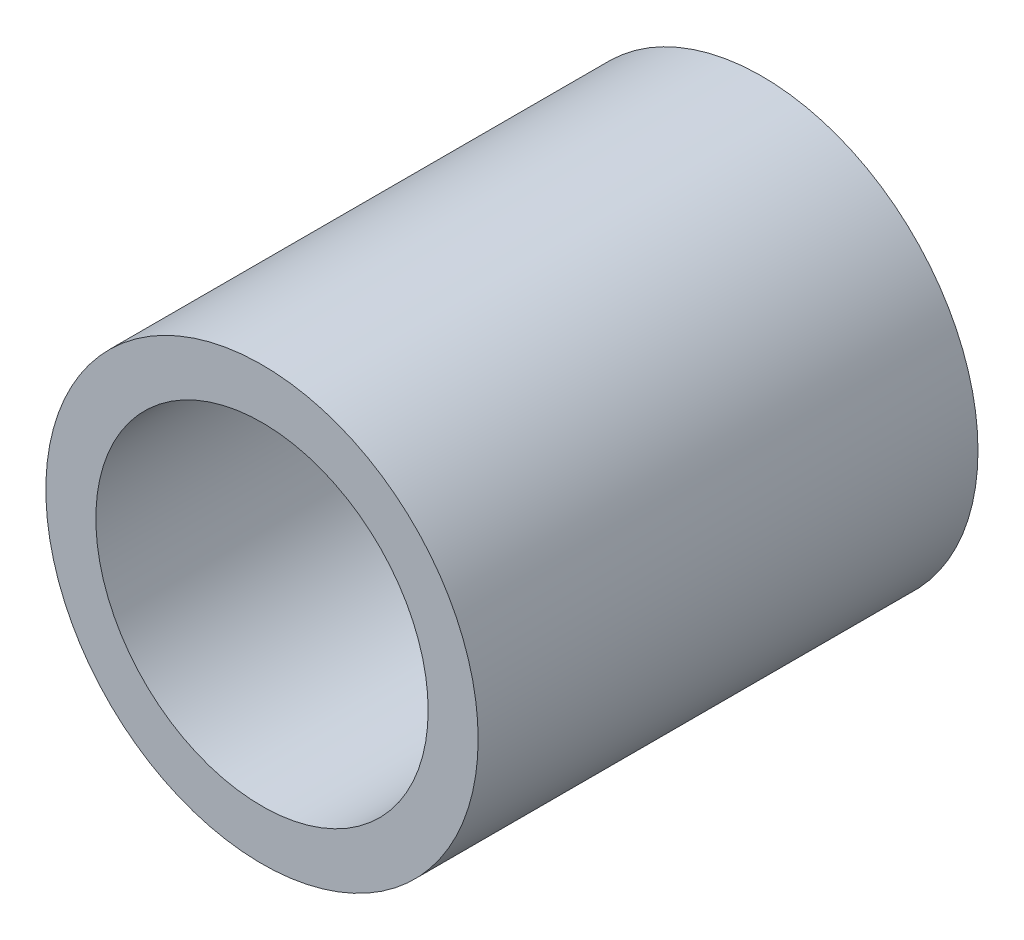
from build123d import *

# Parameters (mm, degrees)
SKETCH1_R           = 8
SKETCH1_R_2         = 6.15
BOSS_EXTRUDE1_DEPTH = 18.5


with BuildPart() as part:
    # Sketch1 → Boss-Extrude1 (new body)
    with BuildSketch(Plane.XY):
        with Locations((100, 71.3)):
            Circle(SKETCH1_R)
        with Locations((100, 71.3)):
            Circle(SKETCH1_R_2, mode=Mode.SUBTRACT)
    extrude(amount=BOSS_EXTRUDE1_DEPTH)


solid = part.part
